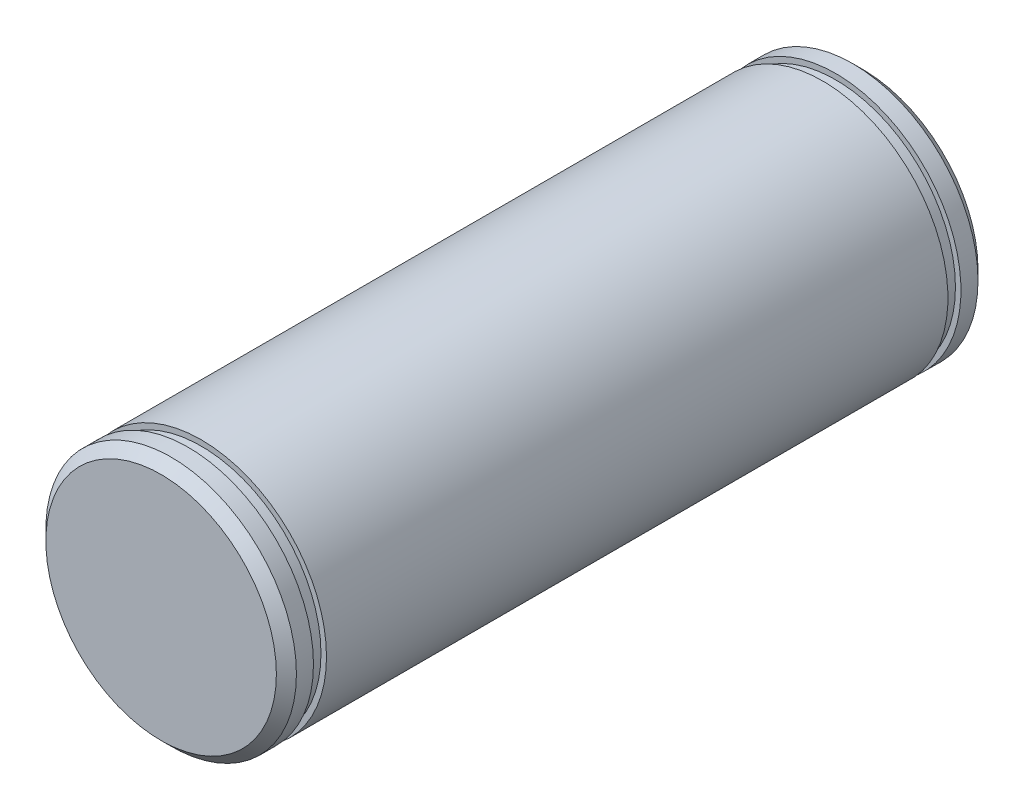
SolidWorks part; units mm, degrees
ref_plane "前视基准面" through (0, 0, 0) normal (0, 0, 1) x (1, 0, 0)
ref_plane "上视基准面" through (0, 0, 0) normal (0, 1, 0) x (1, 0, 0)
ref_plane "右视基准面" through (0, 0, 0) normal (1, 0, 0) x (0, 0, -1)
sketch "草图1" plane through (0, 0, 0) normal (0, 0, 1) x (1, 0, 0)
  circle A0 centre (0, 0) radius 12.5
  dimension "D1" = 25
extrude "凸台-拉伸1" add sketch "草图1" along normal mid plane 70
sketch "草图2" plane through (-0.381, 4.4181, -35) normal (0, 0, -1) x (-1, 0, 0)
  line L0 (-0.381, -4.4181) -> (12.119, -4.4181) construction
  circle A0 centre (-0.381, -4.4181) radius 12.5
  circle A2 centre (-0.381, -4.4181) radius 12.5 construction
  point P2 (12.119, -4.4181)
  dimension "D1" = 25
ref_plane "基准面1" through (-12.5, 0, -35) normal (0, 1, 0) x (1, 0, 0)
sketch "草图3" plane through (-100, 0, -35) normal (0, 1, 0) x (0, 0, 1)
  line L0 (0, 100) -> (33.5023, 100) construction
  line L2 (2.7, 87.5) -> (4, 87.5)
  line L3 (2.7, 87.5) -> (2.7, 88.05)
  line L4 (2.7, 88.05) -> (4, 88.05)
  line L5 (4, 87.5) -> (4, 88.05)
  line L6 (0, 112.5) -> (0, 87.5) construction
  dimension "D1" = 1.3
  dimension "D2" = 11.95
  dimension "D3" = 4
revolve "切除-旋转1" cut sketch "草图3" angle 360 about L0
other "轴卡簧特征库<1>"
sketch "草图21" plane through (6.6624, -2.9033, 35) normal (0, 0, 1) x (1, 0, 0)
  line L0 (-6.6624, 2.9033) -> (5.8376, 2.9033) construction
  circle A0 centre (-6.6624, 2.9033) radius 12.5
  circle A2 centre (-6.6624, 2.9033) radius 12.5 construction
  point P2 (5.8376, 2.9033)
  dimension "D1" = 25
ref_plane "基准面11" through (12.5, 0, 35) normal (0, 1, 0) x (1, 0, 0)
sketch "草图31" plane through (100, 0, 35) normal (0, 1, 0) x (0, 0, -1)
  line L0 (0, 100) -> (33.5023, 100) construction
  line L2 (2.7, 87.5) -> (4, 87.5)
  line L3 (2.7, 87.5) -> (2.7, 88.05)
  line L4 (2.7, 88.05) -> (4, 88.05)
  line L5 (4, 87.5) -> (4, 88.05)
  line L6 (0, 112.5) -> (0, 87.5) construction
  dimension "D1" = 1.3
  dimension "D2" = 11.95
  dimension "D3" = 4
revolve "切除-旋转11" cut sketch "草图31" angle 360 about L0
other "轴卡簧特征库<2>"
chamfer "倒角1" distance 1 angle 45 2 edges at (12.5, 0, 35) (12.5, 0, -35)
